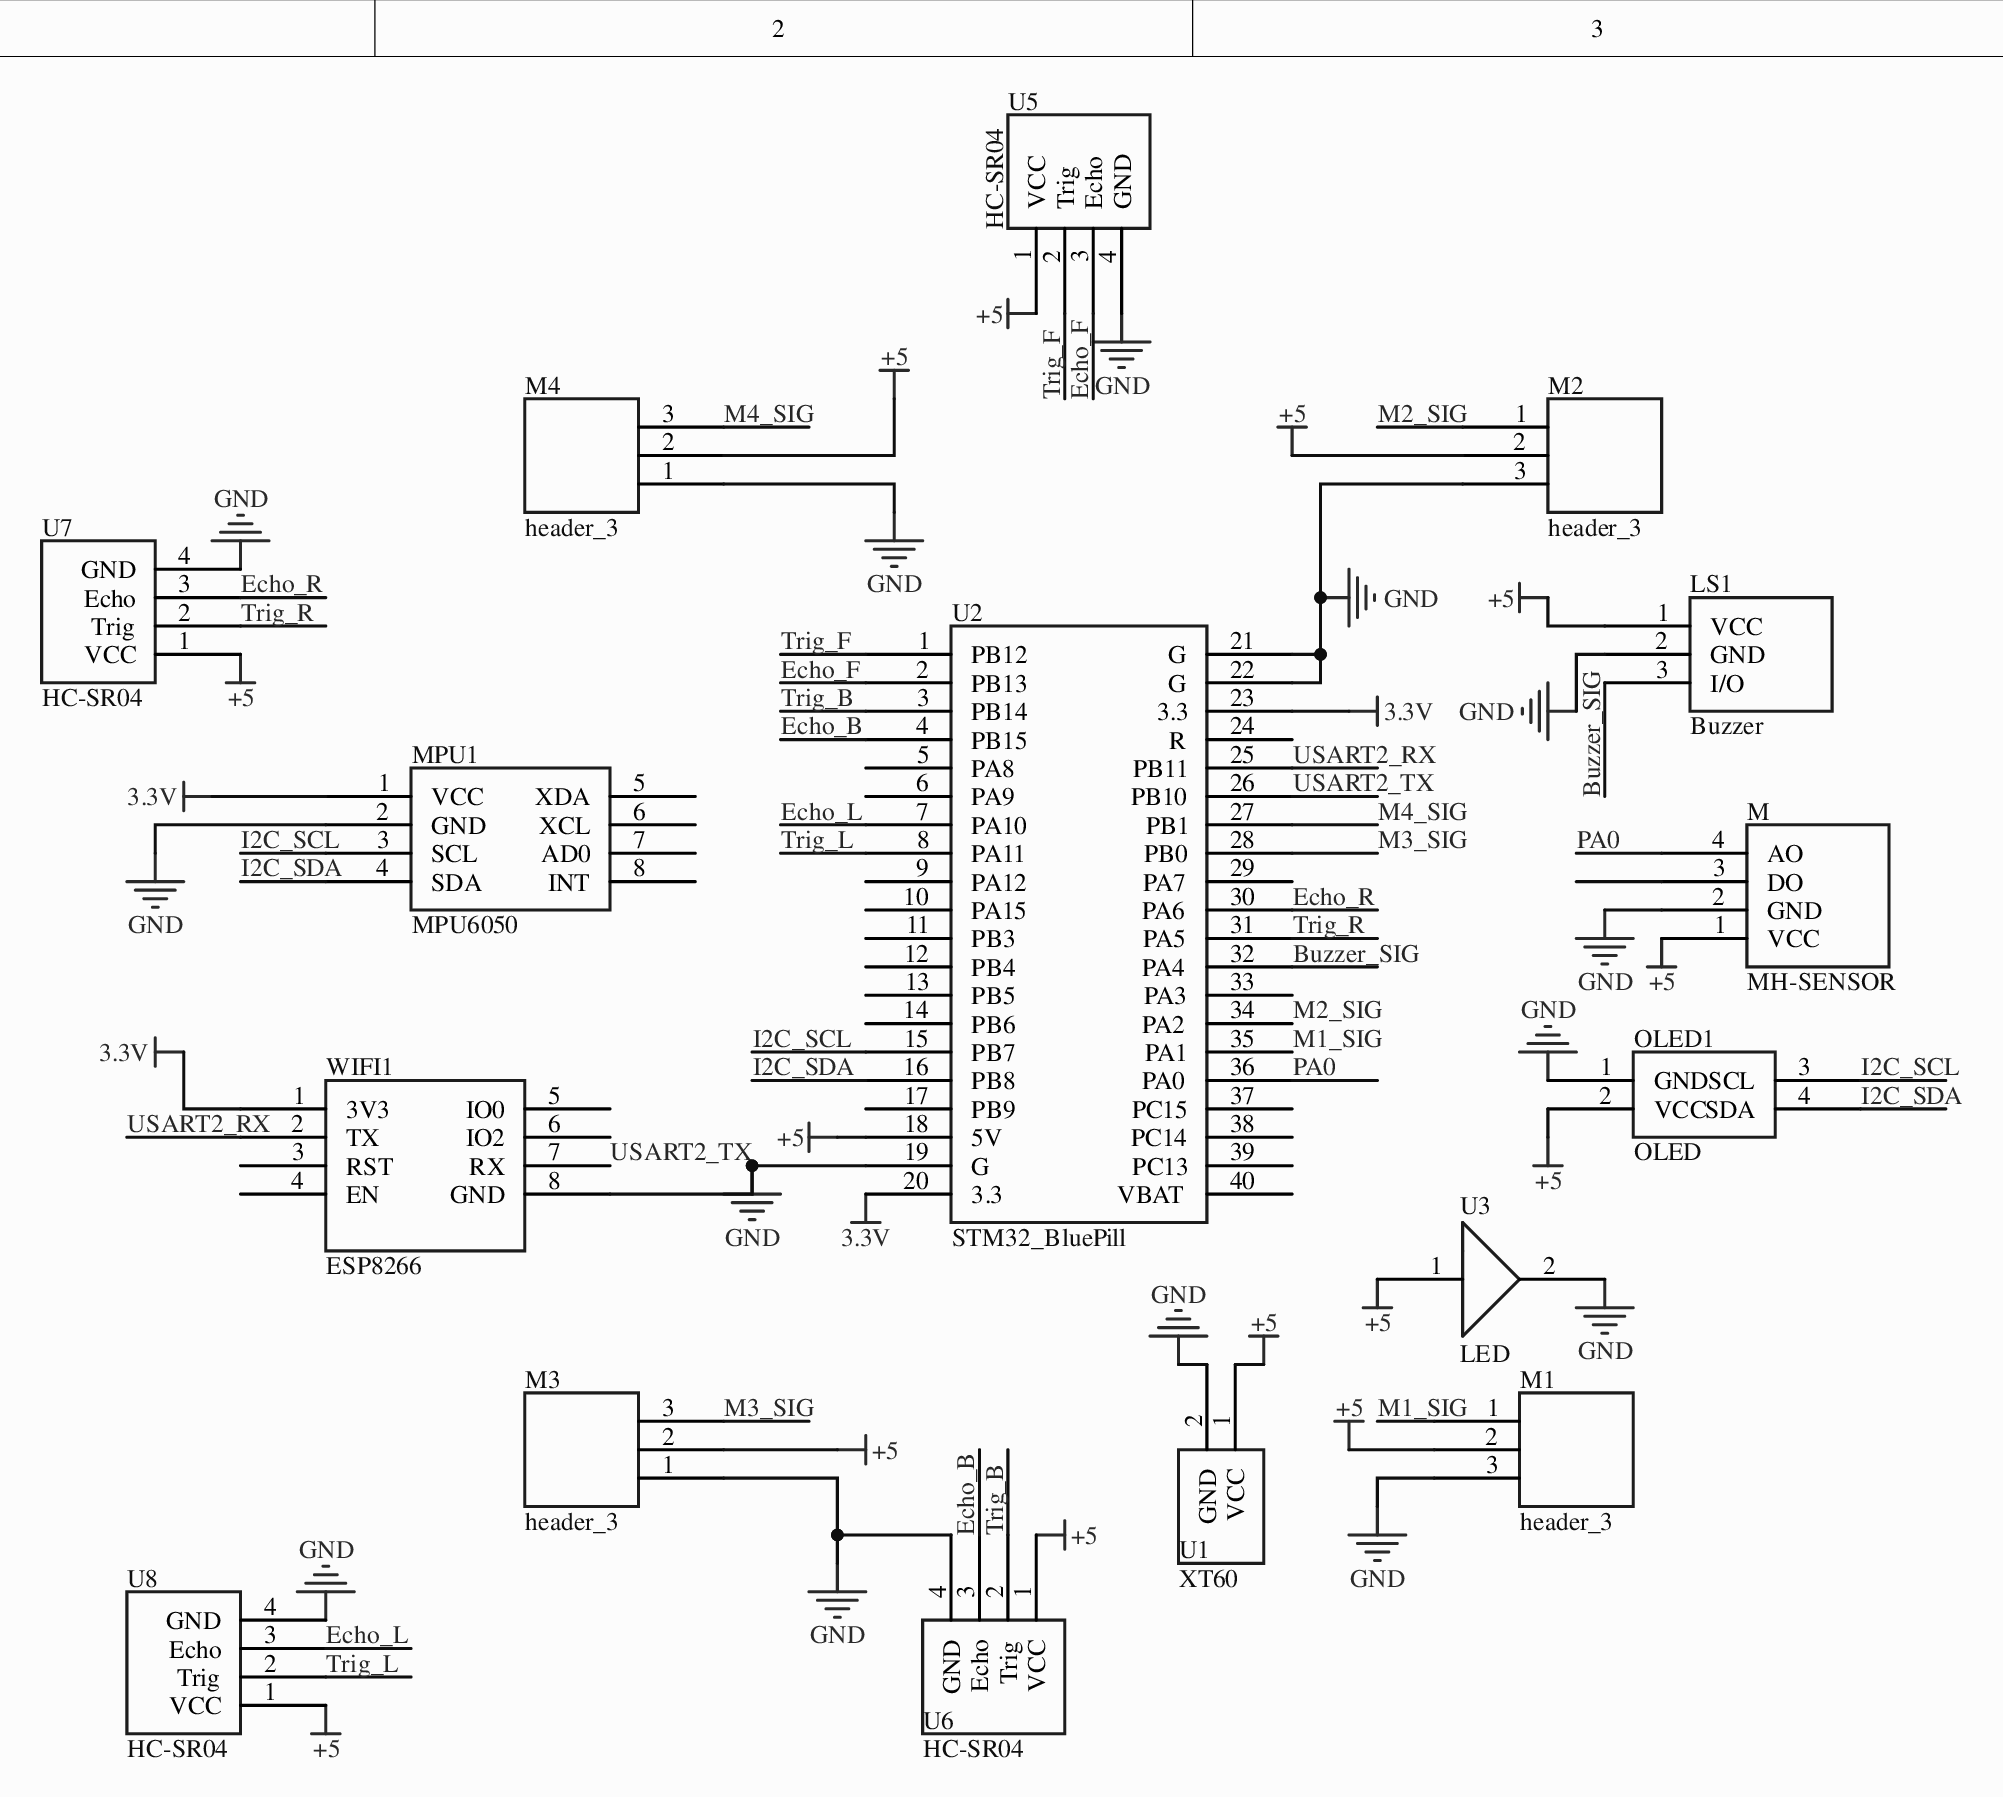
[diagram p0: MISC51067-3.schdoc]
# Altium project MISC51067-2.PrjPcb
1 sheet, 16 parts. Net scope: global (net labels, ports and power ports of the same name join across sheets).
Board file: MISC51067.pcbdoc

## Sheet MISC51067-3.schdoc
size 292 x 193 mm; SheetNumber: 1; SheetTotal: 1; Name: MISC51067

### Parts
LS1  Buzzer  [header]
M  MH-SENSOR  [OLED]
M1  header_3  [header]
M2  header_3  [header]
M3  header_3  [header]
M4  header_3  [header]
MPU1  MPU6050  [MPU6050]
OLED1  OLED  [OLED]
U1  XT60  [XT60]
U2  STM32_BluePill  [STM32_BluePill_1]
U3  LED  [XT60]
U5  HC-SR04  [OLED]
U6  HC-SR04  [OLED]
U7  HC-SR04  [OLED]
U8  HC-SR04  [OLED]
WIFI1  ESP8266  [ESP8266]

### Nets
3.3V: MPU1.1(VCC) U2.20(3.3) U2.23(3.3) WIFI1.1(3V3)
+5: LS1.1(VCC) M.1(VCC) M1.2 M2.2 M3.2 M4.2 OLED1.2(VCC) U1.1(VCC) U2.18(5V) U3.1 U5.1(VCC) U6.1(VCC) U7.1(VCC) U8.1(VCC)
GND: LS1.2(GND) M.2(GND) M1.3 M2.3 M3.1 M4.1 MPU1.2(GND) OLED1.1(GND) U1.2(GND) U2.19(G) U2.21(G) U2.22(G) U3.2 U5.4(GND) U6.4(GND) U7.4(GND) U8.4(GND) WIFI1.8(GND)
Buzzer_SIG: LS1.3(I/O) U2.32(PA4)
Echo_B: U2.4(PB15) U6.3(Echo)
Echo_F: U2.2(PB13) U5.3(Echo)
Echo_L: U2.7(PA10) U8.3(Echo)
Echo_R: U2.30(PA6) U7.3(Echo)
I2C_SCL: MPU1.3(SCL) OLED1.3(SCL) U2.15(PB7)
I2C_SDA: MPU1.4(SDA) OLED1.4(SDA) U2.16(PB8)
M1_SIG: M1.1 U2.35(PA1)
M2_SIG: M2.1 U2.34(PA2)
M3_SIG: M3.3 U2.28(PB0)
M4_SIG: M4.3 U2.27(PB1)
PA0: M.4(AO) U2.36(PA0)
Trig_B: U2.3(PB14) U6.2(Trig)
Trig_F: U2.1(PB12) U5.2(Trig)
Trig_L: U2.8(PA11) U8.2(Trig)
Trig_R: U2.31(PA5) U7.2(Trig)
USART2_RX: U2.25(PB11) WIFI1.2(TX)
USART2_TX: U2.26(PB10) WIFI1.7(RX)

Not connected (* = marked no-connect by the designer): M 3(DO); MPU1 5(XDA) 6(XCL) 7(AD0) 8(INT); U2 5(PA8) 6(PA9) 9(PA12) 10(PA15) 11(PB3) 12(PB4) 13(PB5) 14(PB6) 17(PB9) 24(R) 29(PA7) 33(PA3) 37(PC15) 38(PC14) 39(PC13) 40(VBAT); WIFI1 3(RST) 4(EN) 5(IO0) 6(IO2)

### Library data of the parts
LS1 = Buzzer: Origin Footprint: Header_3; OriginFootprint 2: header3; UniqueId: b3ab9d4e85ca72a5; AddInBom: yes; Device: Buzzer; DesignItemID: Buzzer; LibraryName: Schlib1; SymbolName: Buzzer; FootprintName: header
M = MH-SENSOR: UniqueId: dcc3ce6d5d8a1361; AddInBom: yes; Device: MH-SENSOR; DesignItemID: MH-SENSOR; LibraryName: Schlib1; SymbolName: MH-SENSOR; FootprintName: OLED
M1 = header_3: Origin Footprint: header3; UniqueId: 20f64733a18c5380; AddInBom: yes; Device: header_3; OriginFootprint 2: header3; DesignItemID: header_3; LibraryName: Schlib1; SymbolName: header_3; FootprintName: header
M2 = header_3: Origin Footprint: header3; UniqueId: 0b67e2366e5b1ba6; AddInBom: yes; Device: header_3; OriginFootprint 2: header3; DesignItemID: header_3; LibraryName: Schlib1; SymbolName: header_3; FootprintName: header
M3 = header_3: Origin Footprint: header3; UniqueId: 4e48eb34ab40b298; AddInBom: yes; Device: header_3; OriginFootprint 2: header3; DesignItemID: header_3; LibraryName: Schlib1; SymbolName: header_3; FootprintName: header
M4 = header_3: Origin Footprint: header3; UniqueId: 60a981ccfcd2d311; AddInBom: yes; Device: header_3; OriginFootprint 2: header3; DesignItemID: header_3; LibraryName: Schlib1; SymbolName: header_3; FootprintName: header
MPU1 = MPU6050_1: UniqueId: 749c824cf9e5383c; AddInBom: yes; Device: MPU6050_1; DesignItemID: MPU6050; LibraryName: Schlib1; SymbolName: MPU6050; FootprintName: MPU6050
OLED1 = OLED_3: UniqueId: 109e16bfe7cb1e05; AddInBom: yes; Device: OLED_3; DesignItemID: OLED; LibraryName: Schlib1; SymbolName: OLED; FootprintName: OLED
U1 = XT60_2: UniqueId: gge1; AddInBom: yes; Device: XT60_2; DesignItemID: XT60; LibraryName: Schlib1; SymbolName: XT60; FootprintName: XT60
U2 = STM32_BluePill: UniqueId: 48f0ae2437312dae; AddInBom: yes; Device: STM32_BluePill; DesignItemID: STM32_BluePill; LibraryName: Schlib1; SymbolName: STM32_BluePill; FootprintName: STM32_BluePill_1
U3 = LED: UniqueId: gge2; AddInBom: yes; Device: LED; DesignItemID: LED; LibraryName: Schlib1; SymbolName: LED; FootprintName: XT60
U5 = HC-SR04: UniqueId: adf583383e4d69d4; AddInBom: yes; ModelId: d459d248281f4140aaafbda3f8c1b0d5; Device: HC-SR04; DesignItemID: HC-SR04; LibraryName: Schlib1; SymbolName: HC-SR04; FootprintName: OLED; ModelName: HC-SR04
U6 = HC-SR04: UniqueId: 124c013cfc851acc; AddInBom: yes; ModelId: d459d248281f4140aaafbda3f8c1b0d5; Device: HC-SR04; DesignItemID: HC-SR04; LibraryName: Schlib1; SymbolName: HC-SR04; FootprintName: OLED; ModelName: HC-SR04
U7 = HC-SR04_1: UniqueId: 4ec783ed4741de1f; AddInBom: yes; Device: HC-SR04_1; DesignItemID: HC-SR04; LibraryName: Schlib1; SymbolName: HC-SR04; FootprintName: OLED
U8 = HC-SR04_1: UniqueId: 484e3008dca2bfa8; AddInBom: yes; Device: HC-SR04_1; DesignItemID: HC-SR04; LibraryName: Schlib1; SymbolName: HC-SR04; FootprintName: OLED
WIFI1 = ESP8266_1: UniqueId: 4c39959fcb55ad55; AddInBom: yes; Device: ESP8266_1; DesignItemID: ESP8266; LibraryName: Schlib1; SymbolName: ESP8266; FootprintName: ESP8266